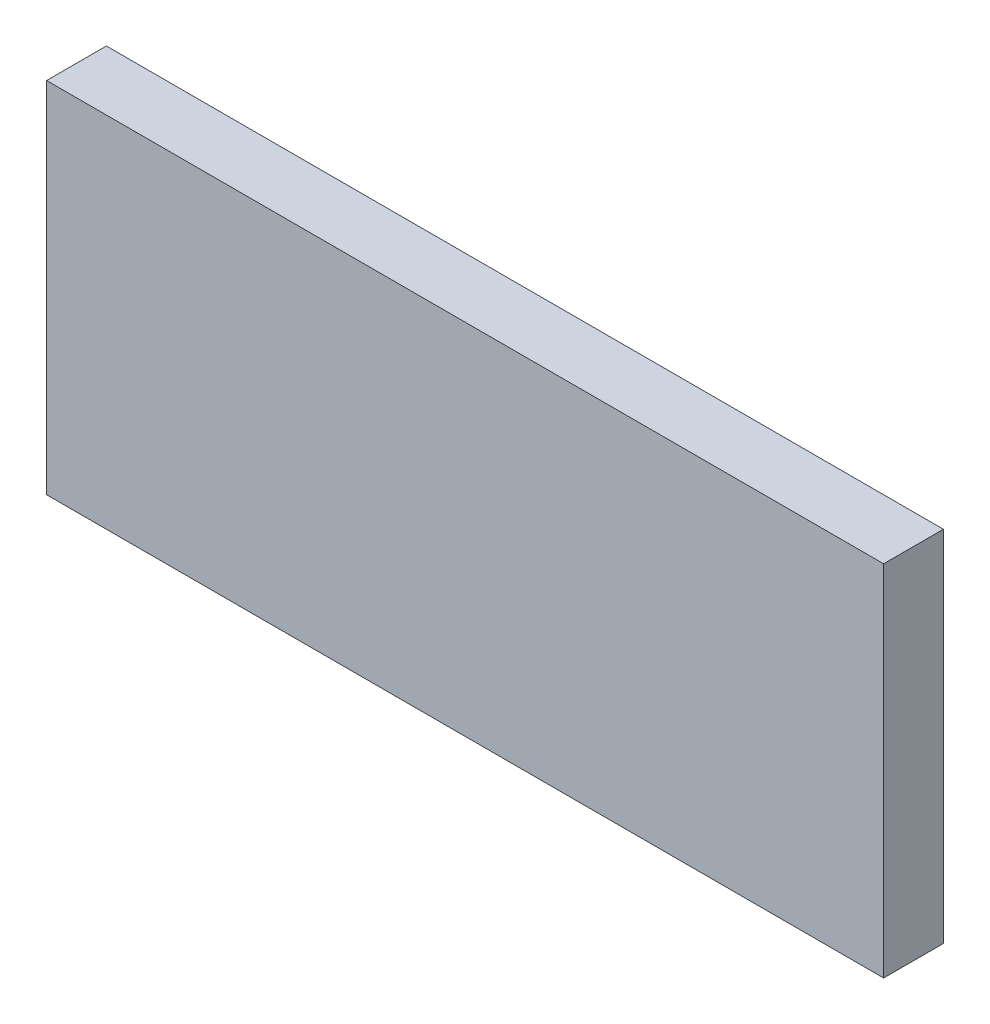
from build123d import *

# Parameters (mm, degrees)
SKETCH_1_W      = 140
SKETCH_1_H      = 60
EXTRUDE_1_DEPTH = 10


with BuildPart() as part:
    # 草图1 → 凸台-拉伸1 (new body)
    with BuildSketch(Plane.XY):
        with Locations((-70, 30)):
            Rectangle(SKETCH_1_W, SKETCH_1_H)
    extrude(amount=EXTRUDE_1_DEPTH)


solid = part.part
